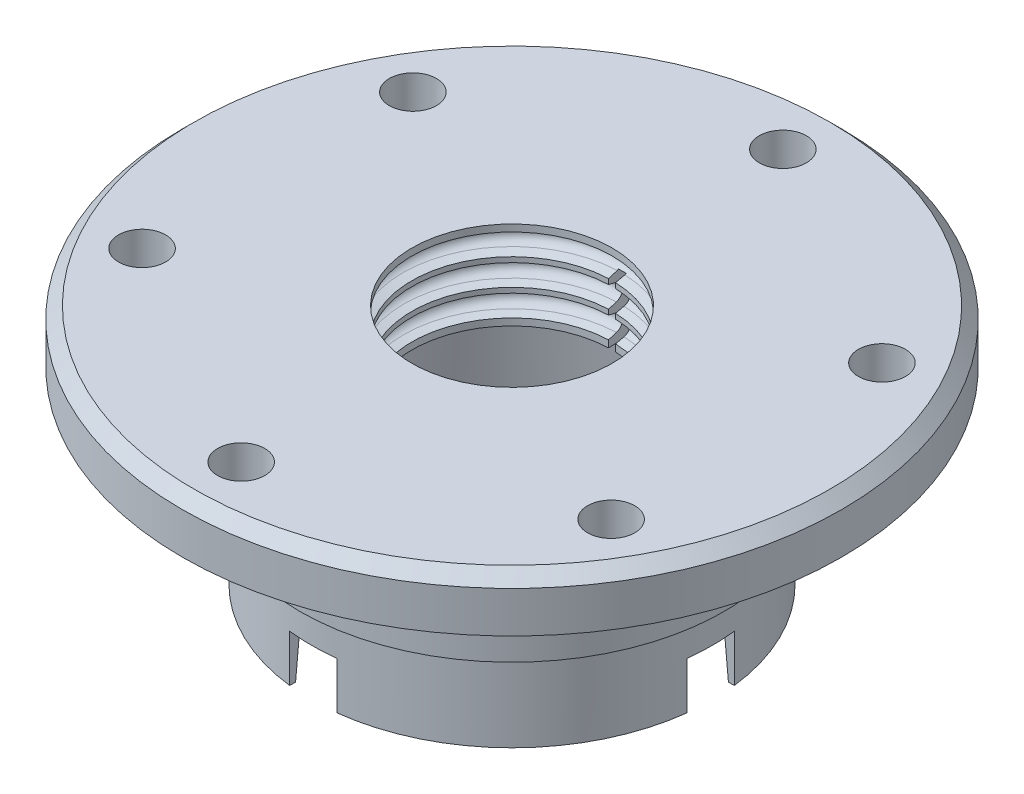
from build123d import *

# Parameters (mm, degrees)
CUT_REVOLVE1_ANGLE = 4.000000000000009
SKETCH4_W          = 37.759390331998226
SKETCH4_H          = 8
CUT_EXTRUDE1_DEPTH = 4
SKETCH5_W          = 44.9966068122979
SKETCH5_H          = 8
CUT_EXTRUDE2_DEPTH = 4
SKETCH6_R          = 4.000000000000005
SKETCH6_R_2        = 4.000000000000001
SKETCH6_R_3        = 3.999999999999999
CUT_EXTRUDE3_DEPTH = 65
SCALE_1_SCALE      = 1.875


with BuildPart() as part:
    # Sketch1 → Revolve1 (revolve)
    with BuildSketch(Plane.XY, mode=Mode.PRIVATE) as revolve1_sk:
        with BuildLine():
            Line((-34, 13.999999999999998), (-34, 0))
            Line((-34, 0), (-33, 0))
            Line((-33, 0), (-30.987496542800134, 21.466703543465286))
            ThreePointArc((-30.987496542800134, 21.466703543465286), (-29.37581336604471, 24.696857971124018), (-26.009325412503696, 25.999999999999996))
            Line((-26.009325412503696, 25.999999999999996), (-17, 25.999999999999996))
            Line((-17, 25.999999999999996), (-17.000000000000004, 27.17913653695376))
            Line((-17.000000000000004, 27.17913653695376), (-18.388228567653776, 27.551111260566394))
            ThreePointArc((-18.388228567653776, 27.551111260566394), (-19.500000000000014, 28.999999999999986), (-18.3882285676538, 30.448888739433595))
            Line((-18.3882285676538, 30.448888739433595), (-17.000000000000007, 30.820863463046255))
            Line((-17.000000000000007, 30.820863463046255), (-17.000000000000007, 31.679136536953756))
            Line((-17.000000000000007, 31.679136536953756), (-18.38822856765378, 32.05111126056639))
            ThreePointArc((-18.38822856765378, 32.05111126056638), (-19.49827813558921, 33.42814856706124), (-18.52509395794485, 34.90508944033103))
            Line((-18.525093957944854, 34.90508944033104), (-17.000000000000007, 35.31373713474397))
            Line((-17.000000000000007, 35.31373713474397), (-17.000000000000007, 36.179136536953735))
            Line((-17.000000000000007, 36.179136536953735), (-17.000000000000004, 36.18626286525602))
            Line((-17.000000000000004, 36.18626286525602), (-18.525093957944854, 36.59491055966894))
            ThreePointArc((-18.525093957944854, 36.59491055966894), (-19.49827813558921, 38.07185143293873), (-18.38822856765378, 39.44888873943359))
            Line((-18.38822856765378, 39.44888873943359), (-17.000000000000007, 39.82086346304622))
            Line((-17.000000000000007, 39.82086346304622), (-17, 40.99999999999999))
            Line((-17, 40.99999999999999), (-54, 40.99999999999999))
            Line((-54, 40.99999999999999), (-56, 39))
            Line((-56, 39), (-56, 32))
            Line((-56, 32), (-34, 31.999999999999993))
            Line((-34, 31.999999999999993), (-34, 29.999999999999993))
            Line((-34, 29.999999999999993), (-36.00000000000001, 29.999999999999993))
            Line((-36.00000000000001, 29.999999999999993), (-36.00000000000001, 13.999999999999998))
            Line((-36.00000000000001, 13.999999999999998), (-34, 13.999999999999998))
        make_face()
    revolve(revolve1_sk.sketch.rotate(Axis((0, 0, 0), (0, 1, 0)), 270), axis=Axis((0, 0, 0), (0, 1, 0)))

    # Sketch3 → Cut-Revolve1 (revolve, symmetric, cut)
    with BuildSketch(Plane(origin=(0, 0, 0), x_dir=(0, 0, -1), z_dir=(1, 0, 0))) as cut_revolve1_sk:
        with BuildLine():
            Line((-17.000000000000014, 32.71643849545569), (-17.000000000000014, 25.999999999999996))
            Line((-17.000000000000014, 25.999999999999996), (-24.215390309173507, 25.999999999999996))
            Line((-24.215390309173507, 25.999999999999996), (-21.000000000000025, 37.99999999999999))
            ThreePointArc((-21.000000000000025, 37.99999999999999), (-19.500000000000025, 36.49999999999999), (-18.00000000000002, 37.99999999999999))
            Line((-18.00000000000002, 37.99999999999999), (-17.000000000000014, 37.99999999999999))
            Line((-17.000000000000014, 37.99999999999999), (-17.000000000000014, 32.71643849545569))
        make_face()
        with BuildLine():
            Line((18.00000000000002, 37.99999999999999), (17.000000000000014, 37.99999999999999))
            Line((17.000000000000014, 37.99999999999999), (17.000000000000014, 32.71643849545569))
            Line((17.000000000000014, 32.71643849545569), (17.000000000000014, 25.999999999999996))
            Line((17.000000000000014, 25.999999999999996), (24.215390309173507, 25.999999999999996))
            Line((24.215390309173507, 25.999999999999996), (21.000000000000025, 37.99999999999999))
            ThreePointArc((21.000000000000025, 37.99999999999999), (19.500000000000025, 36.49999999999999), (18.00000000000002, 37.99999999999999))
        make_face()
    revolve(axis=Axis((0, 0, 0), (0, 1, 0)), revolution_arc=CUT_REVOLVE1_ANGLE / 2, mode=Mode.SUBTRACT)
    revolve(cut_revolve1_sk.sketch, axis=Axis((0, 0, 0), (0, -1, 0)), revolution_arc=CUT_REVOLVE1_ANGLE / 2, mode=Mode.SUBTRACT)

    # Sketch4 → Cut-Extrude1 (cut, symmetric)
    with BuildSketch(Plane(origin=(0, 0, 0), x_dir=(0, 0, -1), z_dir=(1, 0, 0))):
        with Locations((31.466158609998526, 4)):
            Rectangle(SKETCH4_W, SKETCH4_H)
        with Locations((-31.466158609998526, 4)):
            Rectangle(SKETCH4_W, SKETCH4_H)
    extrude(amount=CUT_EXTRUDE1_DEPTH, both=True, mode=Mode.SUBTRACT)

    # Sketch5 → Cut-Extrude2 (cut, symmetric)
    with BuildSketch(Plane.XY):
        with Locations((33.35412812659844, 4)):
            Rectangle(SKETCH5_W, SKETCH5_H)
        with Locations((-33.35412812659844, 4)):
            Rectangle(SKETCH5_W, SKETCH5_H)
    extrude(amount=CUT_EXTRUDE2_DEPTH, both=True, mode=Mode.SUBTRACT)

    # Sketch6 → Cut-Extrude3 (cut)
    with BuildSketch(Plane.XZ):
        with Locations(Location((-39.837168574084245, -22.9999999999999, 0), (0, 0, 270))):
            Circle(SKETCH6_R)
        with Locations(Location((0, 46, 0), (0, 0, 270))):
            Circle(SKETCH6_R_2)
        with Locations(Location((39.837168574084224, 22.999999999999908, 0), (0, 0, 270))):
            Circle(SKETCH6_R_3)
        with Locations(Location((-39.837168574084245, 22.9999999999999, 0), (0, 0, 270))):
            Circle(SKETCH6_R)
        with Locations(Location((0, -46, 0), (0, 0, 270))):
            Circle(SKETCH6_R_2)
        with Locations(Location((39.837168574084224, -22.999999999999908, 0), (0, 0, 270))):
            Circle(SKETCH6_R_3)
    extrude(amount=-CUT_EXTRUDE3_DEPTH, mode=Mode.SUBTRACT)


with BuildPart() as part_1:
    # Scale 1: scaled about (0, 32.2473532, 0)
    add(part.part.scale(SCALE_1_SCALE).moved(Location((0, -28.21643405, 0))))


solid = part_1.part
